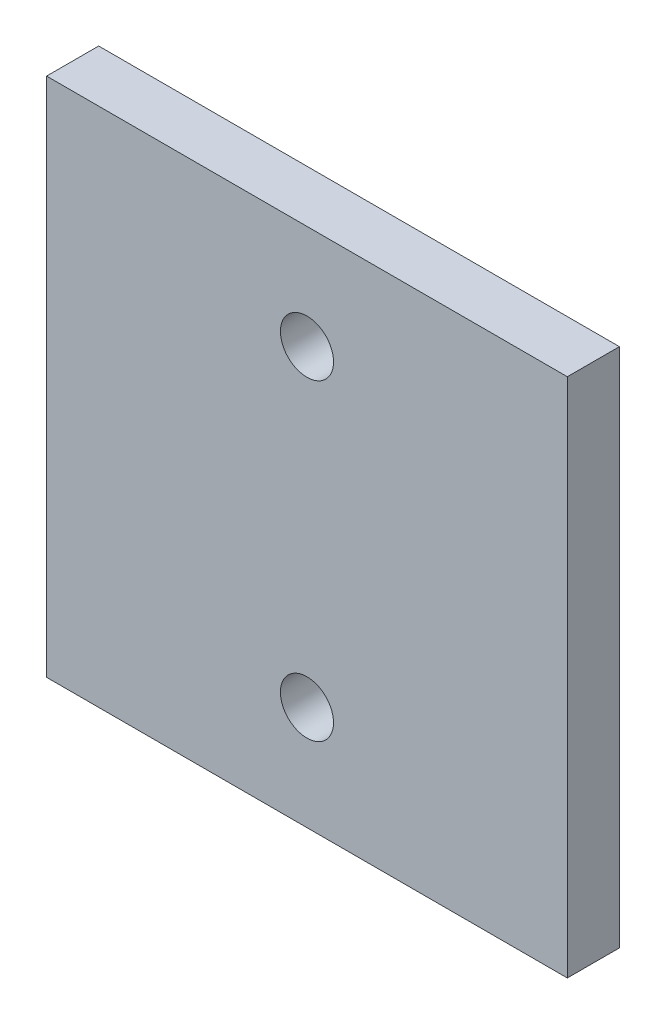
SolidWorks part; units mm, degrees
material "1023 碳钢板 (SS)"
ref_plane "Front Plane" through (0, 0, 0) normal (0, 0, 1) x (1, 0, 0)
ref_plane "Top Plane" through (0, 0, 0) normal (0, 1, 0) x (1, 0, 0)
ref_plane "Right Plane" through (0, 0, 0) normal (1, 0, 0) x (0, 0, -1)
sketch "Sketch1" plane through (0, 0, 0) normal (0, 0, 1) x (1, 0, 0)
  line L1 (50, 50) -> (-50, 50)
  line L2 (50, 50) -> (50, -50)
  line L3 (50, -50) -> (-50, -50)
  line L4 (-50, 50) -> (-50, -50)
  line L5 (50, 50) -> (-50, -50) construction
  line L6 (50, -50) -> (-50, 50) construction
  point P0 (0, 0)
  dimension "D1" = 100
  dimension "D2" = 100
extrude "Boss-Extrude1" add sketch "Sketch1" along normal blind 10
sketch "Sketch2" plane through (0, 0, 10) normal (0, 0, 1) x (1, 0, 0)
  circle A0 centre (0, 30) radius 5.8595
  circle A1 centre (0, -30) radius 6.9059
  dimension "D1" = 60
  dimension "D2" = 30
hole_wizard "M12 Tapped Hole1" positions "Sketch3" profile "Sketch4" tap size "M12" standard "ISO"
sketch "Sketch3" plane through (0, 0, 10) normal (0, 0, 1) x (1, 0, 0)
  point P0 (0, 30)
  point P3 (0, -30)
sketch "Sketch4" plane through (0, 30, 10) normal (1, 0, 0) x (0, -1, 0)
  line L0 (0, 0) -> (0, 32.3144)
  line L1 (0, 32.3144) -> (5.1, 29.25)
  line L2 (5.1, 29.25) -> (5.1, 0)
  line L5 (5.1, 0) -> (0, 0)
  line L10 (0, 32.3144) -> (-5.1, 29.25) construction
  line L11 (0, -6.35) -> (0, 107.95) construction
  dimension "螺纹孔钻头直径" = 10.2
  dimension "螺纹孔钻头深度" = 29.25
  dimension "导头角度" = 118
cosmetic thread "Hole Thread Line 1"
cosmetic thread "Hole Thread Line 2"
